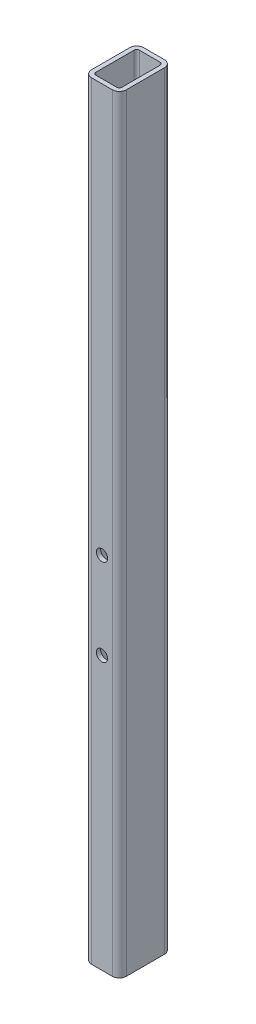
from build123d import *

# Parameters (mm, degrees)
GB_T_6728_2002_RECTANGULAR_HOLLOW_SECTIO_DEPTH = 884
F_13_0_13_DIAMETER_HOLE1_D                     = 13


with BuildPart() as part:
    # Sketch14 → GB/T 6728-2002 rectangular hollow section 60X40X5(1) (new body)
    with BuildSketch(Plane(origin=(0, 0, 0), x_dir=(-1, 0, 0), z_dir=(0, 1, 0))):
        with BuildLine():
            Line((-12, -30), (12, -30))
            ThreePointArc((12, -30), (17.656854249, -27.656854249), (20, -22))
            Line((20, -22), (20, 22))
            ThreePointArc((20, 22), (17.656854249, 27.656854249), (12, 30))
            Line((12, 30), (-12, 30))
            ThreePointArc((-12, 30), (-17.656854249, 27.656854249), (-20, 22))
            Line((-20, 22), (-20, -22))
            ThreePointArc((-20, -22), (-17.656854249, -27.656854249), (-12, -30))
        make_face()
        with BuildLine():
            Line((-12, -25), (12, -25))
            ThreePointArc((12, -25), (14.121320344, -24.121320344), (15, -22))
            Line((15, -22), (15, 22))
            ThreePointArc((15, 22), (14.121320344, 24.121320344), (12, 25))
            Line((12, 25), (-12, 25))
            ThreePointArc((-12, 25), (-14.121320344, 24.121320344), (-15, 22))
            Line((-15, 22), (-15, -22))
            ThreePointArc((-15, -22), (-14.121320344, -24.121320344), (-12, -25))
        make_face(mode=Mode.SUBTRACT)
    extrude(amount=GB_T_6728_2002_RECTANGULAR_HOLLOW_SECTIO_DEPTH)

    # Ø13.0 (13) Diameter Hole1 (through all)
    with Locations(Plane.XY.offset(30)):
        with Locations((0, 414), (0, 314)):
            Hole(F_13_0_13_DIAMETER_HOLE1_D / 2)


solid = part.part
